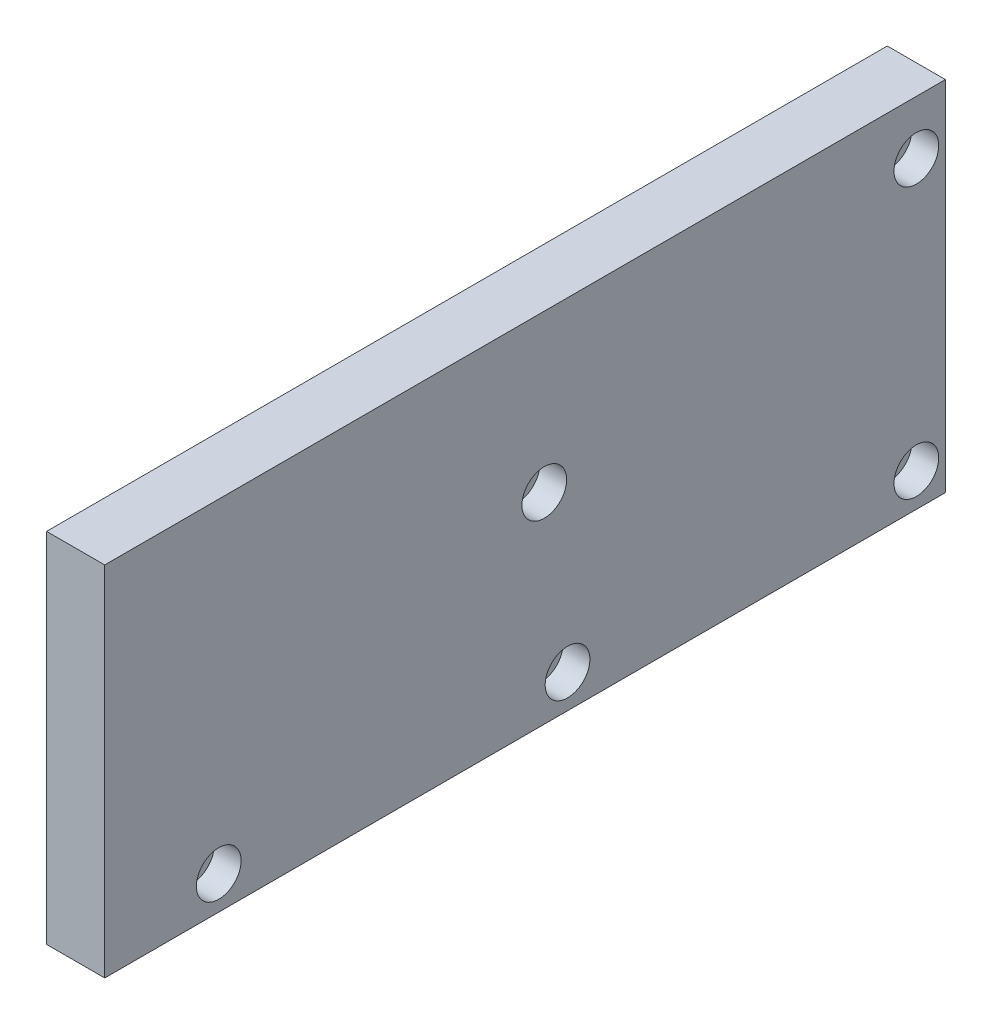
from build123d import *

# Parameters (mm, degrees)
SKETCH1_W           = 188
SKETCH1_H           = 80
BOSS_EXTRUDE1_DEPTH = 13
SKETCH3_R           = 5
SKETCH3_R_2         = 3
CUT_EXTRUDE1_DEPTH  = 6
CUT_EXTRUDE2_REACH  = 104.981
SKETCH3_3_R         = 3
SKETCH4_R           = 5
SKETCH4_R_2         = 3
CUT_EXTRUDE3_DEPTH  = 6
CUT_EXTRUDE4_REACH  = 104.981
SKETCH4_3_R         = 3
SKETCH5_R           = 5
SKETCH5_R_2         = 3
CUT_EXTRUDE5_DEPTH  = 6
CUT_EXTRUDE6_REACH  = 104.981
SKETCH5_3_R         = 3


with BuildPart() as part:
    # Sketch1 → Boss-Extrude1 (new body)
    with BuildSketch(Plane(origin=(0, 0, 0), x_dir=(0, 0, -1), z_dir=(1, 0, 0))):
        Rectangle(SKETCH1_W, SKETCH1_H)
    extrude(amount=BOSS_EXTRUDE1_DEPTH)

    # Sketch3 → Cut-Extrude1 (cut)
    with BuildSketch(Plane(origin=(13, 0, 0), x_dir=(0, 0, -1), z_dir=(1, 0, 0))):
        with Locations((4.3, 4.893325501)):
            Circle(SKETCH3_R)
        with Locations((4.3, 4.893325501)):
            Circle(SKETCH3_R_2, mode=Mode.SUBTRACT)
    extrude(amount=-CUT_EXTRUDE1_DEPTH, mode=Mode.SUBTRACT)

    # Sketch3<3> → Cut-Extrude2 (cut, up to next)
    with BuildSketch(Plane(origin=(13, 0, 0), x_dir=(0, 0, -1), z_dir=(1, 0, 0)), mode=Mode.PRIVATE) as cut_extrude2_sk1:
        with Locations((4.3, 4.893325501)):
            Circle(SKETCH3_3_R)
    cut_extrude2_tool1 = extrude(cut_extrude2_sk1.sketch, amount=-CUT_EXTRUDE2_REACH, mode=Mode.PRIVATE) & part.part
    add(cut_extrude2_tool1.solids().sort_by_distance((13, 4.893326, -4.3))[0], mode=Mode.SUBTRACT)

    # Sketch4 → Cut-Extrude3 (cut)
    # profile 1 of 3: a face of its own
    with BuildSketch(Plane(origin=(13, 0, 0), x_dir=(0, 0, -1), z_dir=(1, 0, 0))):
        with Locations((-68.5, -32.5)):
            Circle(SKETCH4_R)
        with Locations((-68.5, -32.5)):
            Circle(SKETCH4_R_2, mode=Mode.SUBTRACT)
    # profile 2 of 3: a face of its own
    with BuildSketch(Plane(origin=(13, 0, 0), x_dir=(0, 0, -1), z_dir=(1, 0, 0))):
        with Locations((9.5, -32.5)):
            Circle(SKETCH4_R)
        with Locations((9.5, -32.5)):
            Circle(SKETCH4_R_2, mode=Mode.SUBTRACT)
    # profile 3 of 3: a face of its own
    with BuildSketch(Plane(origin=(13, 0, 0), x_dir=(0, 0, -1), z_dir=(1, 0, 0))):
        with Locations((87.5, -32.5)):
            Circle(SKETCH4_R)
        with Locations((87.5, -32.5)):
            Circle(SKETCH4_R_2, mode=Mode.SUBTRACT)
    extrude(amount=-CUT_EXTRUDE3_DEPTH, mode=Mode.SUBTRACT)

    # Sketch4<3> → Cut-Extrude4 (cut, up to next)
    with BuildSketch(Plane(origin=(13, 0, 0), x_dir=(0, 0, -1), z_dir=(1, 0, 0)), mode=Mode.PRIVATE) as cut_extrude4_sk1:
        with Locations((-68.5, -32.5)):
            Circle(SKETCH4_3_R)
    cut_extrude4_tool1 = extrude(cut_extrude4_sk1.sketch, amount=-CUT_EXTRUDE4_REACH, mode=Mode.PRIVATE) & part.part
    # Sketch4<3> → Cut-Extrude4 (cut, up to next)
    with BuildSketch(Plane(origin=(13, 0, 0), x_dir=(0, 0, -1), z_dir=(1, 0, 0)), mode=Mode.PRIVATE) as cut_extrude4_sk2:
        with Locations((9.5, -32.5)):
            Circle(SKETCH4_3_R)
    cut_extrude4_tool2 = extrude(cut_extrude4_sk2.sketch, amount=-CUT_EXTRUDE4_REACH, mode=Mode.PRIVATE) & part.part
    # Sketch4<3> → Cut-Extrude4 (cut, up to next)
    with BuildSketch(Plane(origin=(13, 0, 0), x_dir=(0, 0, -1), z_dir=(1, 0, 0)), mode=Mode.PRIVATE) as cut_extrude4_sk3:
        with Locations((87.5, -32.5)):
            Circle(SKETCH4_3_R)
    cut_extrude4_tool3 = extrude(cut_extrude4_sk3.sketch, amount=-CUT_EXTRUDE4_REACH, mode=Mode.PRIVATE) & part.part
    add(cut_extrude4_tool1.solids().sort_by_distance((13, -32.5, 68.5))[0], mode=Mode.SUBTRACT)
    add(cut_extrude4_tool2.solids().sort_by_distance((13, -32.5, -9.5))[0], mode=Mode.SUBTRACT)
    add(cut_extrude4_tool3.solids().sort_by_distance((13, -32.5, -87.5))[0], mode=Mode.SUBTRACT)

    # Sketch5 → Cut-Extrude5 (cut)
    with BuildSketch(Plane(origin=(13, 0, 0), x_dir=(0, 0, -1), z_dir=(1, 0, 0))):
        with Locations((87.5, 28)):
            Circle(SKETCH5_R)
        with Locations((87.5, 28)):
            Circle(SKETCH5_R_2, mode=Mode.SUBTRACT)
    extrude(amount=-CUT_EXTRUDE5_DEPTH, mode=Mode.SUBTRACT)

    # Sketch5<3> → Cut-Extrude6 (cut, up to next)
    with BuildSketch(Plane(origin=(13, 0, 0), x_dir=(0, 0, -1), z_dir=(1, 0, 0)), mode=Mode.PRIVATE) as cut_extrude6_sk1:
        with Locations((87.5, 28)):
            Circle(SKETCH5_3_R)
    cut_extrude6_tool1 = extrude(cut_extrude6_sk1.sketch, amount=-CUT_EXTRUDE6_REACH, mode=Mode.PRIVATE) & part.part
    add(cut_extrude6_tool1.solids().sort_by_distance((13, 28, -87.5))[0], mode=Mode.SUBTRACT)


solid = part.part
